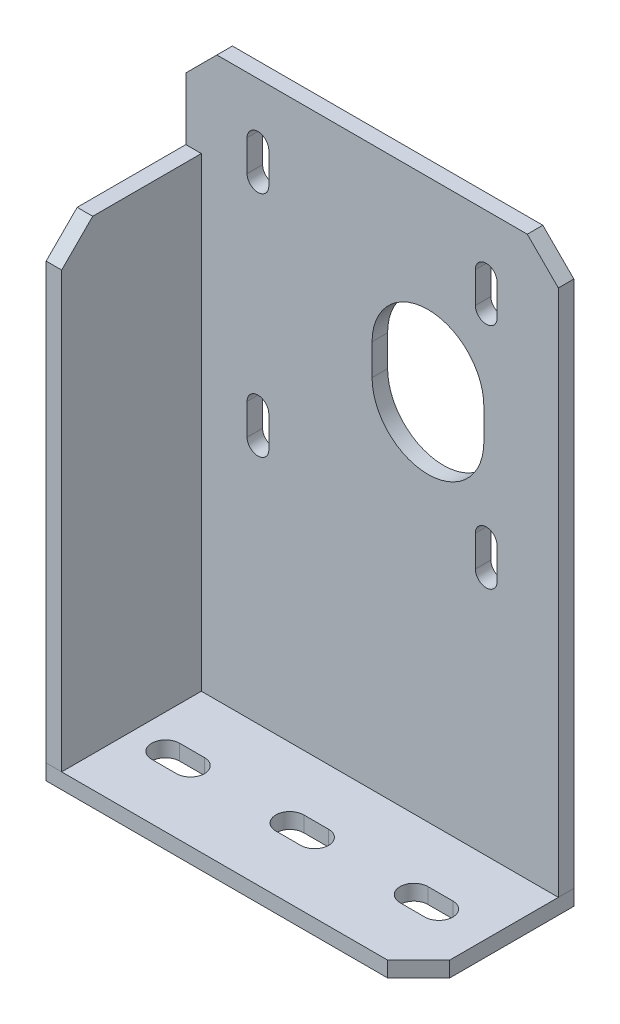
from build123d import *

# Parameters (mm, degrees)
SKETCH_1_W          = 120
SKETCH_1_H          = 50
EXTRUDE_1_DEPTH     = 5
SKETCH_2_W          = 120
SKETCH_2_H          = 5
EXTRUDE_2_DEPTH     = 180
CUT_EXTRUDE_1_DEPTH = 150
CHAMFER_1_SIZE      = 10
SKETCH_5_W          = 45
SKETCH_5_H          = 150
EXTRUDE_3_DEPTH     = 5
CHAMFER_2_SIZE      = 10
SKETCH_6_W          = 80
SKETCH_6_H          = 15
EXTRUDE_4_DEPTH     = 20
CUT_EXTRUDE_2_DEPTH = 20
CHAMFER_3_SIZE      = 10
SKETCH_10_R         = 4.5
CUT_EXTRUDE_3_DEPTH = 20


with BuildPart() as part:
    # 草图1 → 凸台-拉伸1 (new body)
    with BuildSketch(Plane(origin=(0, 0, 0), x_dir=(1, 0, 0), z_dir=(0, 1, 0))):
        Rectangle(SKETCH_1_W, SKETCH_1_H)
    extrude(amount=EXTRUDE_1_DEPTH)

    # 草图9 → 切除-拉伸2 (cut)
    with BuildSketch(Plane(origin=(0, 5, 0), x_dir=(1, 0, 0), z_dir=(0, 1, 0))):
        with BuildLine():
            Line((-44, 2), (-36, 2))
            ThreePointArc((-36, 2), (-31.5, -2.5), (-36, -7))
            Line((-36, -7), (-44, -7))
            ThreePointArc((-44, -7), (-48.5, -2.5), (-44, 2))
        make_face()
        with BuildLine():
            Line((-4, 2), (4, 2))
            ThreePointArc((4, 2), (8.5, -2.5), (4, -7))
            Line((4, -7), (-4, -7))
            ThreePointArc((-4, -7), (-8.5, -2.5), (-4, 2))
        make_face()
        with BuildLine():
            Line((36, 2), (44, 2))
            ThreePointArc((44, 2), (48.5, -2.5), (44, -7))
            Line((44, -7), (36, -7))
            ThreePointArc((36, -7), (31.5, -2.5), (36, 2))
        make_face()
    extrude(amount=-CUT_EXTRUDE_2_DEPTH, mode=Mode.SUBTRACT)

    # 倒角3
    chamfer_3_edges = [part.edges().sort_by_distance(p)[0] for p in [
        (60, 2.5, 25),
    ]]
    chamfer(chamfer_3_edges, length=CHAMFER_3_SIZE)


with BuildPart() as body_2:
    # 草图2 → 凸台-拉伸2 (new body)
    with BuildSketch(Plane(origin=(0, 5, 0), x_dir=(1, 0, 0), z_dir=(0, 1, 0))):
        with Locations((0, 22.5)):
            Rectangle(SKETCH_2_W, SKETCH_2_H)
    extrude(amount=EXTRUDE_2_DEPTH)

    # 草图3 → 切除-拉伸1 (cut)
    with BuildSketch(Plane.XY.offset(-20)):
        with BuildLine():
            Line((-40.269552622, 83.230447378), (-40.269552622, 93.230447378))
            ThreePointArc((-40.269552622, 93.230447378), (-36.769552622, 96.730447378), (-33.269552622, 93.230447378))
            Line((-33.269552622, 93.230447378), (-33.269552622, 83.230447378))
            ThreePointArc((-33.269552622, 83.230447378), (-36.769552622, 79.730447378), (-40.269552622, 83.230447378))
        make_face()
        with BuildLine():
            Line((33.269552622, 83.230447378), (33.269552622, 93.230447378))
            ThreePointArc((33.269552622, 93.230447378), (36.769552622, 96.730447378), (40.269552622, 93.230447378))
            Line((40.269552622, 93.230447378), (40.269552622, 83.230447378))
            ThreePointArc((40.269552622, 83.230447378), (36.769552622, 79.730447378), (33.269552622, 83.230447378))
        make_face()
        with BuildLine():
            Line((33.269552622, 156.769552622), (33.269552622, 166.769552622))
            ThreePointArc((33.269552622, 166.769552622), (36.769552622, 170.269552622), (40.269552622, 166.769552622))
            Line((40.269552622, 166.769552622), (40.269552622, 156.769552622))
            ThreePointArc((40.269552622, 156.769552622), (36.769552622, 153.269552622), (33.269552622, 156.769552622))
        make_face()
        with BuildLine():
            Line((-40.269552622, 156.769552622), (-40.269552622, 166.769552622))
            ThreePointArc((-40.269552622, 166.769552622), (-36.769552622, 170.269552622), (-33.269552622, 166.769552622))
            Line((-33.269552622, 166.769552622), (-33.269552622, 156.769552622))
            ThreePointArc((-33.269552622, 156.769552622), (-36.769552622, 153.269552622), (-40.269552622, 156.769552622))
        make_face()
        with BuildLine():
            Line((0, 120), (0, 130))
            ThreePointArc((0, 130), (18, 148), (36, 130))
            Line((36, 130), (36, 120))
            ThreePointArc((36, 120), (18, 102), (0, 120))
        make_face()
    extrude(amount=-CUT_EXTRUDE_1_DEPTH, mode=Mode.SUBTRACT)

    # 倒角1
    chamfer_1_edges = [body_2.edges().sort_by_distance(p)[0] for p in [
        (60, 185, -22.5),
        (-60, 185, -22.5),
    ]]
    chamfer(chamfer_1_edges, length=CHAMFER_1_SIZE)

    # 草图6 → 凸台-拉伸4 (add)
    with BuildSketch(Plane(origin=(0, 0, -25), x_dir=(-1, 0, 0), z_dir=(0, 0, -1))):
        with Locations((0, 35)):
            Rectangle(SKETCH_6_W, SKETCH_6_H)
    extrude(amount=EXTRUDE_4_DEPTH)

    # 草图10 → 切除-拉伸3 (cut)
    with BuildSketch(Plane.XZ.offset(-27.5)):
        with Locations(Location((-25, -35, 0), (0, 0, 270))):
            Circle(SKETCH_10_R)
        with Locations(Location((25, -35, 0), (0, 0, 270))):
            Circle(SKETCH_10_R)
    extrude(amount=-CUT_EXTRUDE_3_DEPTH, mode=Mode.SUBTRACT)


with BuildPart() as body_3:
    # 草图5 → 凸台-拉伸3 (new body)
    with BuildSketch(Plane.ZY.offset(60)):
        with Locations((2.5, 80)):
            Rectangle(SKETCH_5_W, SKETCH_5_H)
    extrude(amount=-EXTRUDE_3_DEPTH)

    # 倒角2
    chamfer_2_edges = [body_3.edges().sort_by_distance(p)[0] for p in [
        (-57.5, 155, 25),
    ]]
    chamfer(chamfer_2_edges, length=CHAMFER_2_SIZE)


solid = Compound([part.part, body_2.part, body_3.part])
